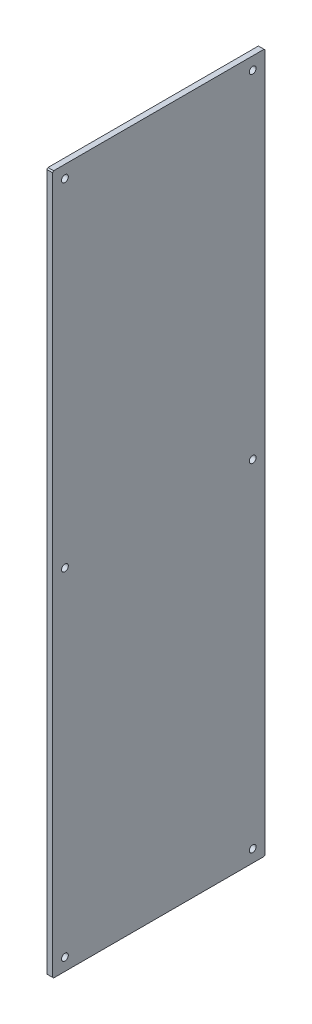
from build123d import *

# Parameters (mm, degrees)
SKETCH_1_W          = 188
SKETCH_1_H          = 618
EXTRUDE_1_DEPTH     = 5
CHAMFER_1_SIZE      = 1
SKETCH_2_R          = 3
CUT_EXTRUDE_1_DEPTH = 324.020123212


with BuildPart() as part:
    # 草图1 → 凸台-拉伸1 (new body)
    with BuildSketch(Plane(origin=(0, 0, 0), x_dir=(0, 0, -1), z_dir=(1, 0, 0))):
        Rectangle(SKETCH_1_W, SKETCH_1_H)
    extrude(amount=EXTRUDE_1_DEPTH)

    # 倒角1
    chamfer_1_edges = [part.edges().sort_by_distance(p)[0] for p in [
        (2.5, 309, 94),
        (2.5, 309, -94),
        (2.5, -309, -94),
        (2.5, -309, 94),
    ]]
    chamfer(chamfer_1_edges, length=CHAMFER_1_SIZE)

    # 草图2 → 切除-拉伸1 (cut, through all)
    with BuildSketch(Plane.ZY):
        with Locations((-83, 298)):
            Circle(SKETCH_2_R)
        with Locations(Location((-83, -298, 0), (0, 0, 180))):
            Circle(SKETCH_2_R)
        with Locations((83, -298)):
            Circle(SKETCH_2_R)
        with Locations(Location((83, 298, 0), (0, 0, 180))):
            Circle(SKETCH_2_R)
        with Locations((83, 0)):
            Circle(SKETCH_2_R)
        with Locations((-83, 0)):
            Circle(SKETCH_2_R)
    extrude(amount=-CUT_EXTRUDE_1_DEPTH, mode=Mode.SUBTRACT)


solid = part.part
